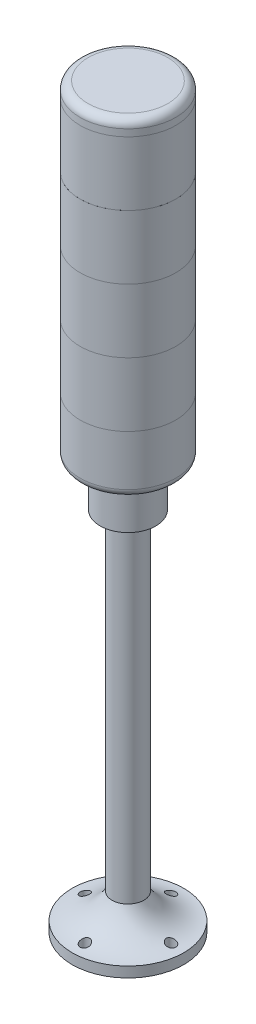
SolidWorks part; units mm, degrees
ref_plane "前视基准面" through (0, 0, 0) normal (0, 0, 1) x (1, 0, 0)
ref_plane "上视基准面" through (0, 0, 0) normal (0, 1, 0) x (1, 0, 0)
ref_plane "右视基准面" through (0, 0, 0) normal (1, 0, 0) x (0, 0, -1)
sketch "草图1" plane through (0, 0, 0) normal (0, 1, 0) x (1, 0, 0)
  circle A0 centre (0, 0) radius 30
  dimension "D1" = 60
extrude "凸台-拉伸1" add sketch "草图1" along normal mid plane 40
sketch "草图2" plane through (0, -20, 0) normal (0, -1, 0) x (1, 0, 0)
  circle A1 centre (0, 0) radius 30
  circle A2 centre (0, 0) radius 30
  dimension "D1" = 0
extrude "凸台-拉伸2" add sketch "草图2" along normal blind 40 separate body
sketch "草图3" plane through (0, -60, 0) normal (0, -1, 0) x (1, 0, 0)
  circle A1 centre (0, 0) radius 30
  circle A2 centre (0, 0) radius 30
  dimension "D1" = 0
extrude "凸台-拉伸3" add sketch "草图3" along normal blind 40 separate body
sketch "草图4" plane through (0, -100, 0) normal (0, -1, 0) x (1, 0, 0)
  circle A1 centre (0, 0) radius 30
  circle A2 centre (0, 0) radius 30
  dimension "D1" = 0
extrude "凸台-拉伸4" add sketch "草图4" along normal blind 40 separate body
sketch "草图5" plane through (0, 20, 0) normal (0, 1, 0) x (1, 0, 0)
  circle A1 centre (0, 0) radius 30
  circle A2 centre (0, 0) radius 30
  dimension "D1" = 0
extrude "凸台-拉伸5" add sketch "草图5" along normal blind 9.35 separate body
sketch "草图6" plane through (0, -140, 0) normal (0, -1, 0) x (1, 0, 0)
  circle A1 centre (0, 0) radius 30
  circle A2 centre (0, 0) radius 30
  dimension "D1" = 0
extrude "凸台-拉伸6" add sketch "草图6" along normal blind 9.35 separate body
sketch "草图7" plane through (0, -149.35, 0) normal (0, -1, 0) x (1, 0, 0)
  circle A1 centre (0, 0) radius 30
  circle A2 centre (0, 0) radius 30
  dimension "D1" = 0
extrude "凸台-拉伸7" add sketch "草图7" along normal blind 27.2
sketch "草图8" plane through (0, -176.55, 0) normal (0, -1, 0) x (1, 0, 0)
  circle A0 centre (0, 0) radius 17.5
  dimension "D1" = 35
extrude "凸台-拉伸8" add sketch "草图8" along normal blind 27.2
fillet "圆角1" radius 5 1 edges at (0, 29.35, 30)
sketch "草图9" plane through (0, -203.75, 0) normal (0, -1, 0) x (1, 0, 0)
  circle A0 centre (0, 0) radius 10
  dimension "D1" = 20
extrude "凸台-拉伸9" add sketch "草图9" along normal blind 207
fillet "圆角2" radius 5 1 edges at (0, -176.55, -17.5)
fillet "圆角3" radius 5 1 edges at (0, -176.55, -30)
sketch "草图10" plane through (0, -410.75, 0) normal (0, -1, 0) x (1, 0, 0)
  circle A0 centre (0, 0) radius 35
  dimension "D1" = 70
extrude "凸台-拉伸10" add sketch "草图10" along normal blind 22.5
sketch "草图11" plane through (0, 0, 0) normal (1, 0, 0) x (0, 0, -1)
  line L0 (35, -433.25) -> (35, -410.75) construction
  line L1 (10, -410.75) -> (35, -410.75)
  line L2 (35, -410.75) -> (-35, -410.75) construction
  line L3 (35, -410.75) -> (35, -426.75)
  line L4 (0, -433.25) -> (0, -389.0111) construction
  line L5 (-35, -433.25) -> (35, -433.25) construction
  arc A0 (10, -410.75) -> (35, -426.75) centre (35.299, -398.7516) ccw
  dimension "D1" = 28
  dimension "D2" = 16
revolve "切除-旋转1" cut sketch "草图11" angle 360 about L4
hole_wizard "Ø6.0 (6) 直径孔2" positions "草图13" profile "草图15" hole size "Ø6.0" standard "ISO"
sketch "草图13" plane through (0, -433.25, 0) normal (0, -1, 0) x (-1, 0, 0)
  circle A0 centre (0, 0) radius 27 construction
  point P5 (0, 27)
  point P7 (27, 0)
  point P9 (-27, 0)
  point P11 (0, -27)
  dimension "D1" = 54
sketch "草图15" plane through (0, -433.25, 27) normal (1, 0, 0) x (0, 0, -1)
  line L0 (0, 0) -> (0, 36.8026)
  line L1 (0, 36.8026) -> (3, 35)
  line L2 (3, 35) -> (3, 0)
  line L5 (3, 0) -> (0, 0)
  line L10 (0, 36.8026) -> (-3, 35) construction
  line L11 (0, -6.35) -> (0, 107.95) construction
  dimension "孔直径" = 6
  dimension "孔深度" = 35
  dimension "导头角度" = 118
